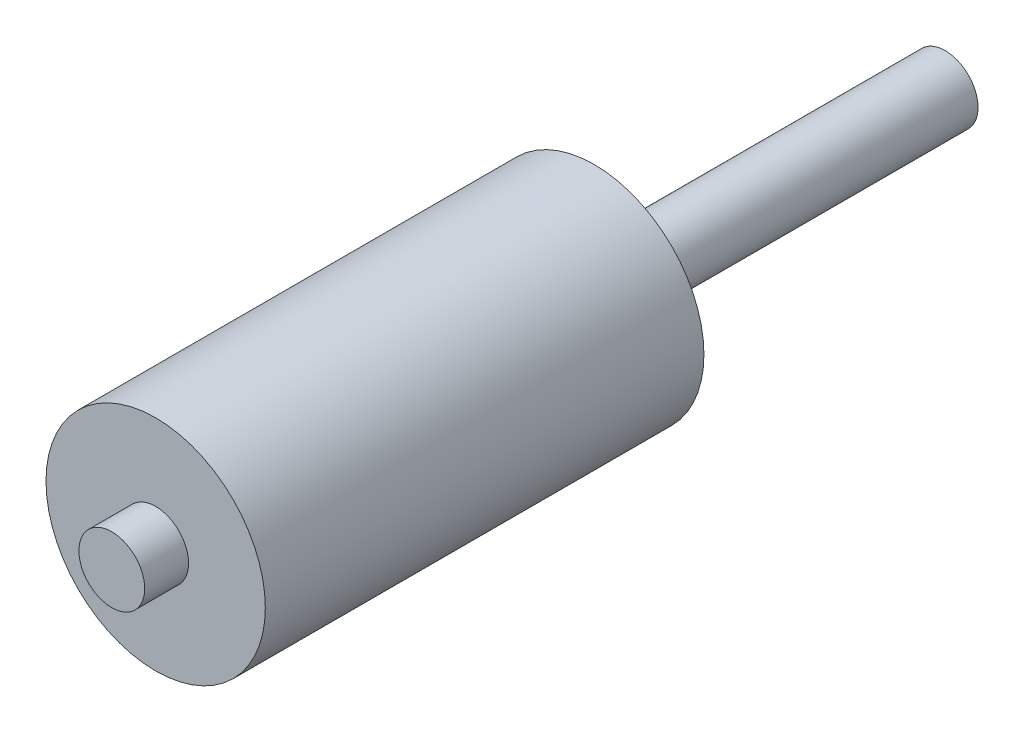
from build123d import *

# Parameters (mm, degrees)
SKETCH_1_R      = 25
EXTRUDE_1_DEPTH = 100
SKETCH_2_R      = 7.5
EXTRUDE_2_DEPTH = 10
EXTRUDE_START   = 80
SKETCH_3_R      = 7.5
EXTRUDE_3_DEPTH = 80


with BuildPart() as part:
    # 草图1 → 凸台-拉伸1 (new body)
    with BuildSketch(Plane.XY):
        Circle(SKETCH_1_R)
    extrude(amount=EXTRUDE_1_DEPTH)

    # 草图2 → 凸台-拉伸2 (add)
    with BuildSketch(Plane.XY.offset(100)):
        Circle(SKETCH_2_R)
    extrude(amount=EXTRUDE_2_DEPTH)

    # 草图3 → 凸台-拉伸3 (add)
    with BuildSketch(Plane(origin=(0, 0, 0), x_dir=(-1, 0, 0), z_dir=(0, 0, -1)).offset(EXTRUDE_START)):
        with Locations(Location((0, 0, 0), (0, 0, 180))):
            Circle(SKETCH_3_R)
    extrude(amount=-EXTRUDE_3_DEPTH)


solid = part.part
